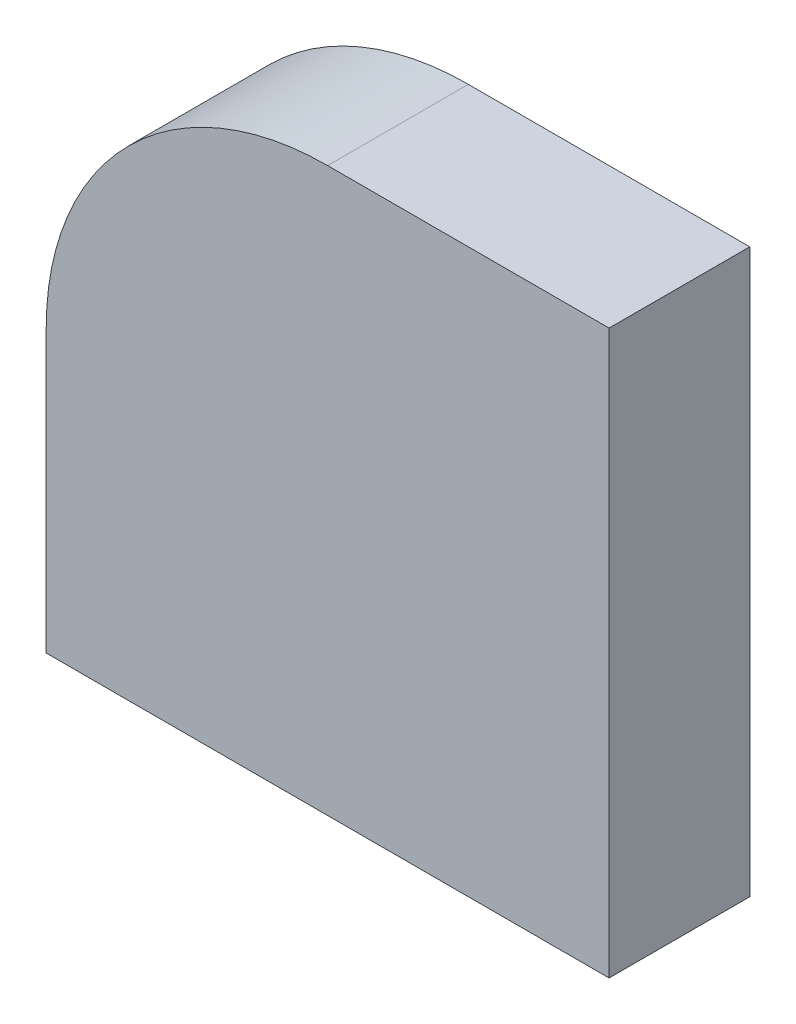
SolidWorks part; units mm, degrees
material "Q235A"
ref_plane "Front Plane" through (0, 0, 0) normal (0, 0, 1) x (1, 0, 0)
ref_plane "Top Plane" through (0, 0, 0) normal (0, 1, 0) x (1, 0, 0)
ref_plane "Right Plane" through (0, 0, 0) normal (1, 0, 0) x (0, 0, -1)
sketch "Sketch1" plane through (0, 0, 0) normal (0, 0, 1) x (1, 0, 0)
  line L0 (0, 0) -> (0, 40)
  line L1 (0, 40) -> (40, 40)
  line L2 (40, 40) -> (40, 0)
  line L5 (40, 0) -> (0, 0)
  dimension "D1" = 40
  dimension "D2" = 40
extrude "Boss-Extrude1" add sketch "Sketch1" along normal blind 10
fillet "Fillet1" radius 20 1 edges at (0, 40, 5)
